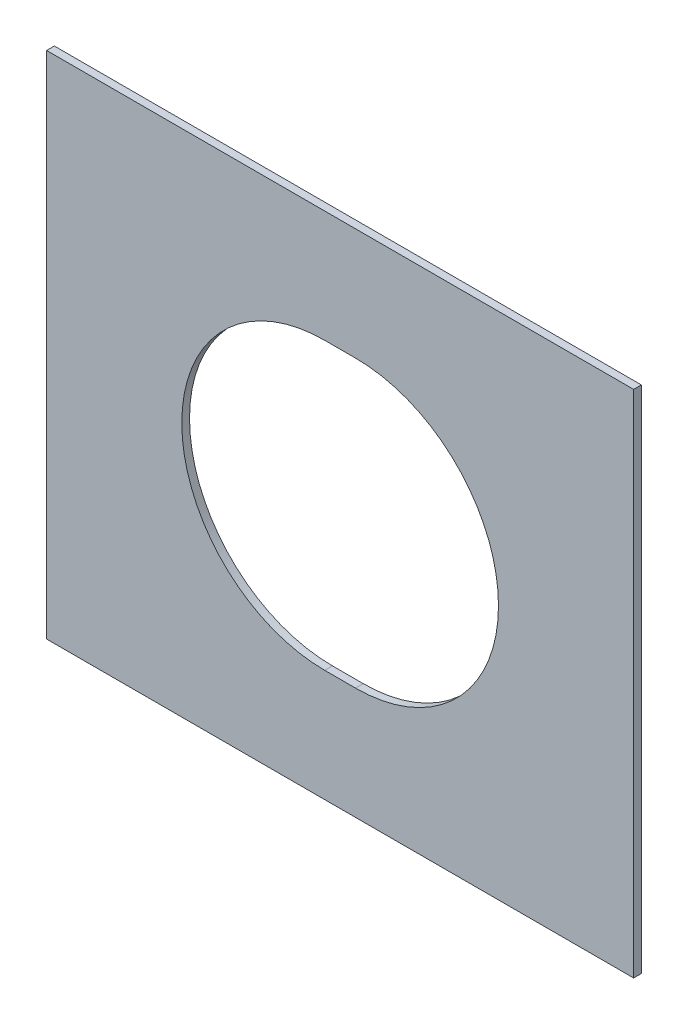
from build123d import *

# Parameters (mm, degrees)
SKETCH_1_W          = 380
SKETCH_1_H          = 330
EXTRUDE_1_DEPTH     = 5
CUT_EXTRUDE_1_DEPTH = 10
EXTRUDE_2_DEPTH     = 5


with BuildPart() as part:
    # 草图1 → 凸台-拉伸1 (new body)
    with BuildSketch(Plane.XY):
        with Locations((190, 165)):
            Rectangle(SKETCH_1_W, SKETCH_1_H)
    extrude(amount=EXTRUDE_1_DEPTH)

    # 草图2 → 切除-拉伸1 (cut)
    with BuildSketch(Plane(origin=(0, 0, 0), x_dir=(-1, 0, 0), z_dir=(0, 0, -1))):
        with BuildLine():
            Line((-210, 72.5), (-170, 72.5))
            ThreePointArc((-170, 72.5), (-77.5, 165), (-170, 257.5))
            Line((-170, 257.5), (-210, 257.5))
            ThreePointArc((-210, 257.5), (-302.5, 165), (-210, 72.5))
        make_face()
    extrude(amount=-CUT_EXTRUDE_1_DEPTH, mode=Mode.SUBTRACT)

    # 草图3 → 凸台-拉伸2 (add)
    with BuildSketch(Plane(origin=(0, 0, 0), x_dir=(-1, 0, 0), z_dir=(0, 0, -1))):
        with BuildLine():
            ThreePointArc((-210, 257.5), (-302.5, 165), (-210, 72.5))
            Line((-210, 72.5), (-200, 72.5))
            ThreePointArc((-200, 72.5), (-292.5, 165), (-200, 257.5))
            Line((-200, 257.5), (-210, 257.5))
        make_face()
        with BuildLine():
            ThreePointArc((-180, 257.5), (-87.5, 165), (-180, 72.5))
            Line((-180, 72.5), (-170, 72.5))
            ThreePointArc((-170, 72.5), (-77.5, 165), (-170, 257.5))
            Line((-170, 257.5), (-180, 257.5))
        make_face()
    extrude(amount=-EXTRUDE_2_DEPTH)


solid = part.part
